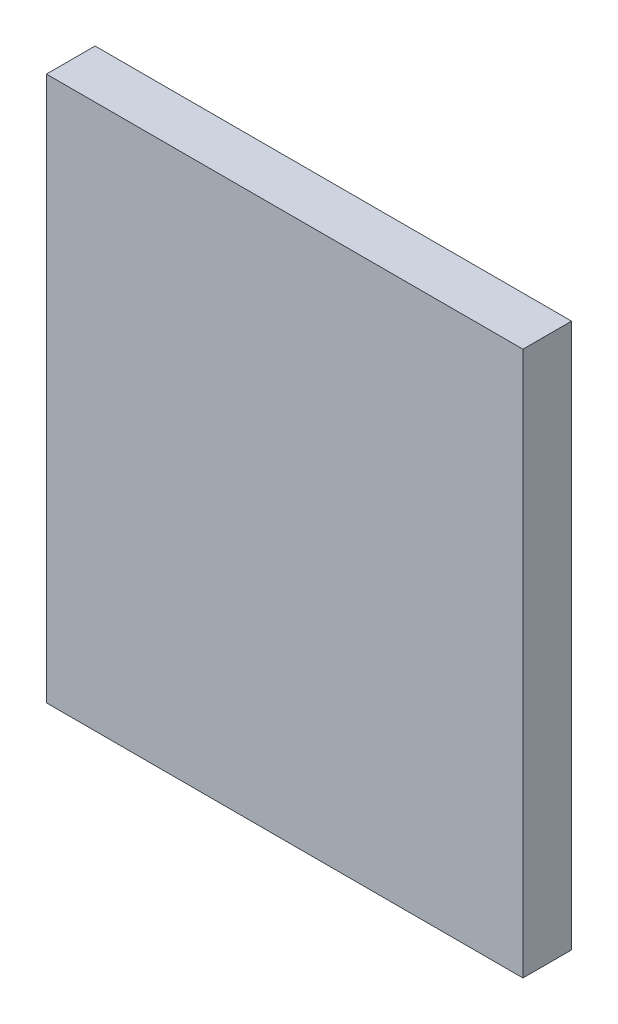
SolidWorks part; units mm, degrees
ref_plane "前视基准面" through (0, 0, 0) normal (0, 0, 1) x (1, 0, 0)
ref_plane "上视基准面" through (0, 0, 0) normal (0, 1, 0) x (1, 0, 0)
ref_plane "右视基准面" through (0, 0, 0) normal (1, 0, 0) x (0, 0, -1)
sketch "草图1" plane through (0, 0, 0) normal (0, 0, 1) x (1, 0, 0)
  line L1 (-122.5, 140) -> (122.5, 140)
  line L2 (-122.5, 140) -> (-122.5, -140)
  line L3 (-122.5, -140) -> (122.5, -140)
  line L4 (122.5, 140) -> (122.5, -140)
  line L5 (-122.5, 140) -> (122.5, -140) construction
  line L6 (-122.5, -140) -> (122.5, 140) construction
  point P0 (0, 0)
  dimension "D1" = 245
  dimension "D2" = 280
extrude "凸台-拉伸1" add sketch "草图1" along normal blind 25
